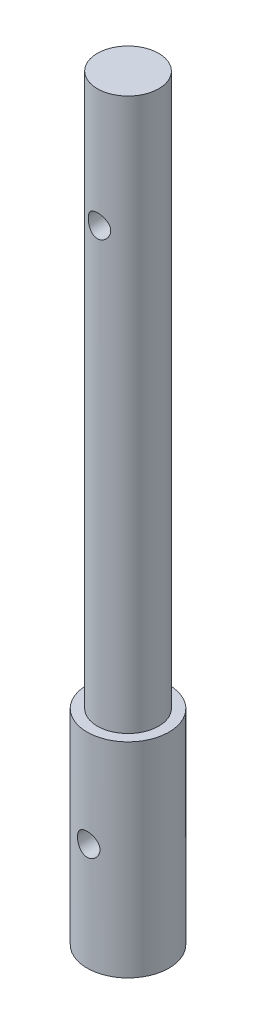
from build123d import *

# Parameters (mm, degrees)
SKETCH_2_R          = 1.1
CUT_EXTRUDE_1_DEPTH = 15


with BuildPart() as part:
    # 草图1 → 旋转1 (revolve)
    with BuildSketch(Plane.XY, mode=Mode.PRIVATE) as revolve_1_sk:
        Polygon((0, 68.097402597), (3, 68.097402597), (3, 14.097402597), (4, 14.097402597), (4, -5.902597403), (0, -5.902597403), align=None)
    revolve(revolve_1_sk.sketch.rotate(Axis((0, 0, 0), (0, 1, 0)), 90), axis=Axis((0, 0, 0), (0, 1, 0)))

    # 草图2 → 切除-拉伸1 (cut, symmetric)
    with BuildSketch(Plane.XY):
        with Locations((0, 56.497402597)):
            Circle(SKETCH_2_R)
        with Locations((0, 4.597402597)):
            Circle(SKETCH_2_R)
    extrude(amount=CUT_EXTRUDE_1_DEPTH, both=True, mode=Mode.SUBTRACT)


solid = part.part
